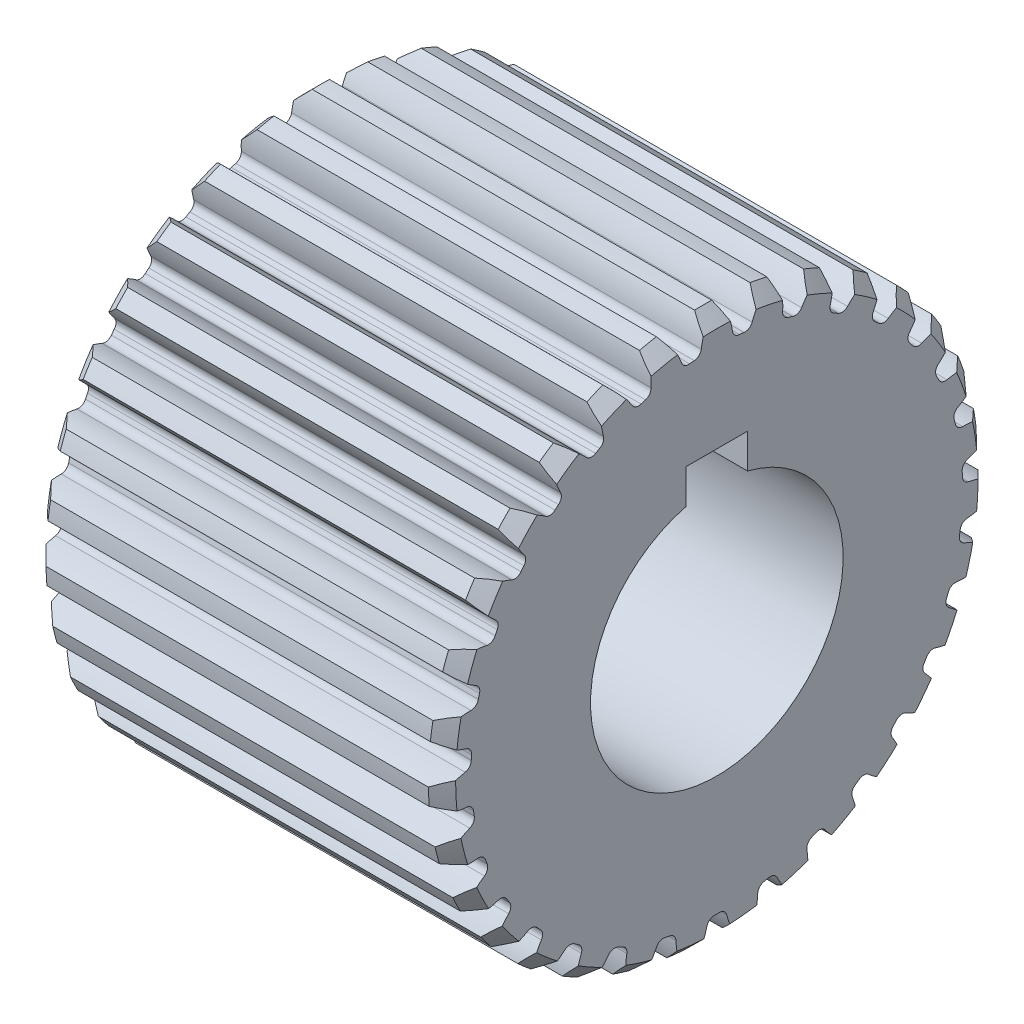
SolidWorks part; units mm, degrees
ref_plane "Front" through (0, 0, 0) normal (0, 0, 1) x (1, 0, 0)
ref_plane "Top" through (0, 0, 0) normal (0, 1, 0) x (1, 0, 0)
ref_plane "Right" through (0, 0, 0) normal (1, 0, 0) x (0, 0, -1)
sketch "Sketch1" plane through (0, 0, 0) normal (0, 0, 1) x (1, 0, 0)
  line L1 (31.1495, 18.25) -> (31.1495, 38.25)
  line L2 (31.1495, 38.25) -> (29.1495, 40.25)
  line L3 (29.1495, 40.25) -> (-26.8505, 40.25)
  line L4 (-26.8505, 40.25) -> (-28.8505, 38.25)
  line L5 (-28.8505, 38.25) -> (-28.8505, 18.25)
  line L6 (-28.8505, 18.25) -> (-28.8505, 0)
  line L7 (-28.8505, 0) -> (31.1495, 0)
  line L8 (31.1495, 0) -> (31.1495, 18.25)
  dimension "D2" = 40.25
  dimension "D3" = 60
  dimension "D4" = 56
  dimension "D5" = 2
  dimension "D6" = 2
  dimension "D7" = 2
revolve "Revolve1" add sketch "Sketch1" angle 360 about L7
sketch "Sketch2" plane through (0, 0, 0) normal (0, 0, 1) x (1, 0, 0)
  line L0 (0, 0) -> (44.1495, 0)
  line L1 (44.1495, 0) -> (44.1495, 19)
  line L2 (44.1495, 19) -> (-36.766, 19)
  line L3 (-36.766, 19) -> (-36.766, 0)
  line L4 (-36.766, 0) -> (0, 0)
  line L5 (0, 0) -> (0.5684, -0.1453)
  dimension "D1" = 19
revolve "Cut-Revolve1" cut sketch "Sketch2" angle 360 about L4
sketch "Sketch3" plane through (-28.8505, 0, 0) normal (-1, 0, 0) x (0, 0, 1)
  circle A0 centre (0, 0) radius 40.25 construction
  circle A1 centre (0, 0) radius 40.25
sketch "Sketch4" plane through (-28.8505, 0, 0) normal (-1, 0, 0) x (0, 0, 1)
  line L0 (0, 0) -> (0, 50.4222) construction
  circle A0 centre (0, 0) radius 40.25 construction
  arc A1 (1.2604, 40.2303) -> (-1.2604, 40.2303) centre (0, 0) ccw
  arc A2 (1.9993, 38.6984) -> (1.8415, 38.7062) centre (0, 0) ccw
  arc A3 (6.8637, 39.6605) -> (5.1716, 36.4916) centre (17.2742, 32.0653) ccw
  arc A4 (1.8415, 38.7062) -> (1.9993, 38.6984) centre (0, 0) cw
  arc A5 (9.3329, 39.153) -> (6.8637, 39.6605) centre (0, 0) ccw
  arc A6 (1.2604, 40.2303) -> (2.2799, 36.7857) centre (-10.4659, 34.8861) cw
  arc A7 (-1.2604, 40.2303) -> (-2.2799, 36.7857) centre (10.4659, 34.8861) ccw
  arc A8 (9.3329, 39.153) -> (9.6382, 35.5737) centre (-3.2291, 36.2788) cw
  arc A9 (3.9794, 35.7794) -> (5.1716, 36.4916) centre (4.1366, 36.8702) ccw
  arc A10 (10.453, 34.449) -> (9.6382, 35.5737) centre (10.7386, 35.5134) cw
  arc A11 (14.7068, 37.4669) -> (12.4115, 34.7036) centre (23.3753, 27.9316) ccw
  arc A12 (17.0233, 36.4729) -> (14.7068, 37.4669) centre (0, 0) ccw
  arc A13 (17.0233, 36.4729) -> (16.6018, 32.9054) centre (4.1398, 36.1862) cw
  arc A14 (11.1002, 34.2459) -> (12.4115, 34.7036) centre (11.4738, 35.2828) ccw
  arc A15 (17.1735, 31.6397) -> (16.6018, 32.9054) centre (17.6676, 32.6248) cw
  arc A16 (21.9478, 33.7395) -> (19.1432, 31.4948) centre (28.5194, 22.6544) ccw
  arc A17 (24.0167, 32.2995) -> (21.9478, 33.7395) centre (0, 0) ccw
  arc A18 (24.0167, 32.2995) -> (22.8858, 28.8899) centre (11.3393, 34.6121) cw
  arc A19 (17.7667, 31.3105) -> (19.1432, 31.4948) centre (18.3413, 32.2509) ccw
  arc A20 (23.191, 27.535) -> (22.8858, 28.8899) centre (23.8733, 28.4005) cw
  arc A21 (28.2903, 28.6308) -> (25.0912, 26.9966) centre (32.4959, 16.4498) ccw
  arc A22 (30.027, 26.8038) -> (28.2903, 28.6308) centre (0, 0) ccw
  arc A23 (30.027, 26.8038) -> (28.2328, 23.6916) centre (18.0746, 31.621) cw
  arc A24 (23.7057, 27.0931) -> (25.0912, 26.9966) centre (24.4579, 27.8986) ccw
  arc A25 (28.259, 22.3031) -> (28.2328, 23.6916) centre (29.1016, 23.0135) cw
  arc A26 (33.4745, 22.35) -> (30.012, 21.3932) centre (35.142, 9.5717) ccw
  arc A27 (34.8079, 20.2108) -> (33.4745, 22.35) centre (0, 0) ccw
  arc A28 (34.8079, 20.2108) -> (32.424, 17.5234) centre (24.0698, 27.3354) cw
  arc A29 (28.6743, 21.7666) -> (30.012, 21.3932) centre (29.5732, 22.4042) ccw
  arc A30 (32.1701, 16.158) -> (32.424, 17.5234) centre (33.1384, 16.6843) cw
  arc A31 (37.2883, 15.1541) -> (33.704, 14.9139) centre (36.3494, 2.3017) ccw
  arc A32 (38.1637, 12.7903) -> (37.2883, 15.1541) centre (0, 0) ccw
  arc A33 (38.1637, 12.7903) -> (35.2877, 10.6378) centre (29.0797, 21.9306) cw
  arc A34 (32.4689, 15.549) -> (33.704, 14.9139) centre (33.4778, 15.9925) ccw
  arc A35 (34.7642, 9.3515) -> (35.2877, 10.6378) centre (35.8186, 9.6721) cw
  arc A36 (39.5755, 7.3378) -> (36.0163, 7.824) centre (36.0687, -5.0625) ccw
  arc A37 (39.9572, 4.8461) -> (39.5755, 7.3378) centre (0, 0) ccw
  arc A38 (39.9572, 4.8461) -> (36.7067, 3.3167) centre (32.899, 15.628) cw
  arc A39 (34.9342, 8.6947) -> (36.0163, 7.824) centre (36.0118, 8.9261) ccw
  arc A40 (35.935, 2.1621) -> (36.7067, 3.3167) centre (37.0324, 2.2638) cw
  arc A41 (40.2425, -0.7789) -> (36.854, 0.4139) centre (34.3113, -12.2194) ccw
  arc A42 (40.1148, -3.2964) -> (40.2425, -0.7789) centre (0, 0) ccw
  arc A43 (40.1148, -3.2964) -> (36.623, -4.1402) centre (35.3715, 8.6855) cw
  arc A44 (35.9694, 1.4845) -> (36.854, 0.4139) centre (37.0714, 1.4943) ccw
  arc A45 (35.6346, -5.1159) -> (36.623, -4.1402) centre (36.73, -5.2371) cw
  arc A46 (39.2619, -8.8637) -> (36.1829, -7.0133) centre (31.1492, -18.8761) ccw
  arc A47 (38.6301, -11.3039) -> (39.2619, -8.8637) centre (0, 0) ccw
  arc A48 (38.6301, -11.3039) -> (35.0399, -11.4276) centre (36.3958, 1.3875) cw
  arc A49 (35.5319, -5.7864) -> (36.1829, -7.0133) centre (36.6134, -5.9987) ccw
  arc A50 (33.8754, -12.1844) -> (35.0399, -11.4276) centre (34.924, -12.5236) cw
  arc A51 (36.674, -16.5856) -> (34.0304, -14.1533) centre (26.7118, -24.76) ccw
  arc A52 (35.5639, -18.8487) -> (36.674, -16.5856) centre (0, 0) ccw
  arc A53 (35.5639, -18.8487) -> (32.0223, -18.2472) centre (35.9301, -5.9673) cw
  arc A54 (33.6398, -12.8205) -> (34.0304, -14.1533) centre (34.6563, -13.2462) ccw
  arc A55 (30.7293, -18.754) -> (32.0223, -18.2472) centre (31.6881, -19.2973) cw
  arc A56 (32.5846, -23.6285) -> (30.4848, -20.7138) centre (21.1809, -29.6302) ccw
  arc A57 (31.0416, -25.6219) -> (32.5846, -23.6285) centre (0, 0) ccw
  arc A58 (31.0416, -25.6219) -> (27.6937, -24.3197) centre (33.9934, -13.0778) cw
  arc A59 (30.3704, -19.3297) -> (30.4848, -20.7138) centre (31.2805, -19.9513) ccw
  arc A60 (26.3251, -24.5559) -> (27.6937, -24.3197) centre (27.1549, -25.2811) cw
  arc A61 (27.1612, -29.7041) -> (25.6911, -26.4264) centre (14.7828, -33.2874) ccw
  arc A62 (25.2486, -31.346) -> (27.1612, -29.7041) centre (0, 0) ccw
  arc A63 (25.2486, -31.346) -> (22.2313, -29.3965) centre (30.665, -19.6529) cw
  arc A64 (25.8577, -25.0476) -> (25.6911, -26.4264) centre (26.624, -25.8396) ccw
  arc A65 (20.8431, -29.3524) -> (22.2313, -29.3965) centre (21.51, -30.2298) cw
  arc A66 (20.6258, -34.5635) -> (19.8456, -31.057) centre (7.7795, -35.5817) ccw
  arc A67 (18.4218, -35.7869) -> (20.6258, -34.5635) centre (0, 0) ccw
  arc A68 (18.4218, -35.7869) -> (15.8587, -33.2699) centre (26.0812, -25.4235) cw
  arc A69 (20.2863, -29.7399) -> (19.8456, -31.057) centre (20.8776, -30.67) ccw
  arc A70 (14.5079, -32.9472) -> (15.8587, -33.2699) centre (14.9845, -33.941) cw
  arc A71 (13.246, -38.008) -> (13.1877, -34.4162) centre (0.4577, -36.4193) ccw
  arc A72 (10.8409, -38.7626) -> (13.246, -38.008) centre (0, 0) ccw
  arc A73 (10.8409, -38.7626) -> (8.8369, -35.7812) centre (20.4296, -30.1531) cw
  arc A74 (13.8845, -33.2148) -> (13.1877, -34.4162) centre (14.2764, -34.2448) ccw
  arc A75 (7.5787, -35.1932) -> (8.8369, -35.7812) centre (7.8455, -36.2625) cw
  arc A76 (5.3239, -39.8963) -> (5.9898, -36.3663) centre (-6.8828, -35.766) ccw
  arc A77 (2.8161, -40.1514) -> (5.3239, -39.8963) centre (0, 0) ccw
  arc A78 (2.8161, -40.1514) -> (1.4533, -36.8276) centre (13.9416, -33.6483) cw
  arc A79 (6.9142, -35.3298) -> (5.9898, -36.3663) centre (7.0907, -36.4176) ccw
  arc A80 (0.3392, -35.9984) -> (1.4533, -36.8276) centre (0.3853, -37.0995) cw
  arc A81 (-2.8161, -40.1514) -> (-1.4533, -36.8276) centre (-13.9416, -33.6483) ccw
  arc A82 (-5.3239, -39.8963) -> (-2.8161, -40.1514) centre (0, 0) ccw
  arc A83 (-5.3239, -39.8963) -> (-5.9898, -36.3663) centre (6.8828, -35.766) cw
  arc A84 (-0.3392, -35.9984) -> (-1.4533, -36.8276) centre (-0.3853, -37.0995) ccw
  arc A85 (-6.9142, -35.3298) -> (-5.9898, -36.3663) centre (-7.0907, -36.4176) cw
  arc A86 (-10.8409, -38.7626) -> (-8.8369, -35.7812) centre (-20.4296, -30.1531) ccw
  arc A87 (-13.246, -38.008) -> (-10.8409, -38.7626) centre (0, 0) ccw
  arc A88 (-13.246, -38.008) -> (-13.1877, -34.4162) centre (-0.4577, -36.4193) cw
  arc A89 (-7.5787, -35.1932) -> (-8.8369, -35.7812) centre (-7.8455, -36.2625) ccw
  arc A90 (-13.8845, -33.2148) -> (-13.1877, -34.4162) centre (-14.2764, -34.2448) cw
  arc A91 (-18.4218, -35.7869) -> (-15.8587, -33.2699) centre (-26.0812, -25.4235) ccw
  arc A92 (-20.6258, -34.5635) -> (-18.4218, -35.7869) centre (0, 0) ccw
  arc A93 (-20.6258, -34.5635) -> (-19.8456, -31.057) centre (-7.7795, -35.5817) cw
  arc A94 (-14.5079, -32.9472) -> (-15.8587, -33.2699) centre (-14.9845, -33.941) ccw
  arc A95 (-20.2863, -29.7399) -> (-19.8456, -31.057) centre (-20.8776, -30.67) cw
  arc A96 (-25.2486, -31.346) -> (-22.2313, -29.3965) centre (-30.665, -19.6529) ccw
  arc A97 (-27.1612, -29.7041) -> (-25.2486, -31.346) centre (0, 0) ccw
  arc A98 (-27.1612, -29.7041) -> (-25.6911, -26.4264) centre (-14.7828, -33.2874) cw
  arc A99 (-20.8431, -29.3524) -> (-22.2313, -29.3965) centre (-21.51, -30.2298) ccw
  arc A100 (-25.8577, -25.0476) -> (-25.6911, -26.4264) centre (-26.624, -25.8396) cw
  arc A101 (-31.0416, -25.6219) -> (-27.6937, -24.3197) centre (-33.9934, -13.0778) ccw
  arc A102 (-32.5846, -23.6285) -> (-31.0416, -25.6219) centre (0, 0) ccw
  arc A103 (-32.5846, -23.6285) -> (-30.4848, -20.7138) centre (-21.1809, -29.6302) cw
  arc A104 (-26.3251, -24.5559) -> (-27.6937, -24.3197) centre (-27.1549, -25.2811) ccw
  arc A105 (-30.3704, -19.3297) -> (-30.4848, -20.7138) centre (-31.2805, -19.9513) cw
  arc A106 (-35.5639, -18.8487) -> (-32.0223, -18.2472) centre (-35.9301, -5.9673) ccw
  arc A107 (-36.674, -16.5856) -> (-35.5639, -18.8487) centre (0, 0) ccw
  arc A108 (-36.674, -16.5856) -> (-34.0304, -14.1533) centre (-26.7118, -24.76) cw
  arc A109 (-30.7293, -18.754) -> (-32.0223, -18.2472) centre (-31.6881, -19.2973) ccw
  arc A110 (-33.6398, -12.8205) -> (-34.0304, -14.1533) centre (-34.6563, -13.2462) cw
  arc A111 (-38.6301, -11.3039) -> (-35.0399, -11.4276) centre (-36.3958, 1.3875) ccw
  arc A112 (-39.2619, -8.8637) -> (-38.6301, -11.3039) centre (0, 0) ccw
  arc A113 (-39.2619, -8.8637) -> (-36.1829, -7.0133) centre (-31.1492, -18.8761) cw
  arc A114 (-33.8754, -12.1844) -> (-35.0399, -11.4276) centre (-34.924, -12.5236) ccw
  arc A115 (-35.5319, -5.7864) -> (-36.1829, -7.0133) centre (-36.6134, -5.9987) cw
  arc A116 (-40.1148, -3.2964) -> (-36.623, -4.1402) centre (-35.3715, 8.6855) ccw
  arc A117 (-40.2425, -0.7789) -> (-40.1148, -3.2964) centre (0, 0) ccw
  arc A118 (-40.2425, -0.7789) -> (-36.854, 0.4139) centre (-34.3113, -12.2194) cw
  arc A119 (-35.6346, -5.1159) -> (-36.623, -4.1402) centre (-36.73, -5.2371) ccw
  arc A120 (-35.9694, 1.4845) -> (-36.854, 0.4139) centre (-37.0714, 1.4943) cw
  arc A121 (-39.9572, 4.8461) -> (-36.7067, 3.3167) centre (-32.899, 15.628) ccw
  arc A122 (-39.5755, 7.3378) -> (-39.9572, 4.8461) centre (0, 0) ccw
  arc A123 (-39.5755, 7.3378) -> (-36.0163, 7.824) centre (-36.0687, -5.0625) cw
  arc A124 (-35.935, 2.1621) -> (-36.7067, 3.3167) centre (-37.0324, 2.2638) ccw
  arc A125 (-34.9342, 8.6947) -> (-36.0163, 7.824) centre (-36.0118, 8.9261) cw
  arc A126 (-38.1637, 12.7903) -> (-35.2877, 10.6378) centre (-29.0797, 21.9306) ccw
  arc A127 (-37.2883, 15.1541) -> (-38.1637, 12.7903) centre (0, 0) ccw
  arc A128 (-37.2883, 15.1541) -> (-33.704, 14.9139) centre (-36.3494, 2.3017) cw
  arc A129 (-34.7642, 9.3515) -> (-35.2877, 10.6378) centre (-35.8186, 9.6721) ccw
  arc A130 (-32.4689, 15.549) -> (-33.704, 14.9139) centre (-33.4778, 15.9925) cw
  arc A131 (-34.8079, 20.2108) -> (-32.424, 17.5234) centre (-24.0698, 27.3354) ccw
  arc A132 (-33.4745, 22.35) -> (-34.8079, 20.2108) centre (0, 0) ccw
  arc A133 (-33.4745, 22.35) -> (-30.012, 21.3932) centre (-35.142, 9.5717) cw
  arc A134 (-32.1701, 16.158) -> (-32.424, 17.5234) centre (-33.1384, 16.6843) ccw
  arc A135 (-28.6743, 21.7666) -> (-30.012, 21.3932) centre (-29.5732, 22.4042) cw
  arc A136 (-30.027, 26.8038) -> (-28.2328, 23.6916) centre (-18.0746, 31.621) ccw
  arc A137 (-28.2903, 28.6308) -> (-30.027, 26.8038) centre (0, 0) ccw
  arc A138 (-28.2903, 28.6308) -> (-25.0912, 26.9966) centre (-32.4959, 16.4498) cw
  arc A139 (-28.259, 22.3031) -> (-28.2328, 23.6916) centre (-29.1016, 23.0135) ccw
  arc A140 (-23.7057, 27.0931) -> (-25.0912, 26.9966) centre (-24.4579, 27.8986) cw
  arc A141 (-24.0167, 32.2995) -> (-22.8858, 28.8899) centre (-11.3393, 34.6121) ccw
  arc A142 (-21.9478, 33.7395) -> (-24.0167, 32.2995) centre (0, 0) ccw
  arc A143 (-21.9478, 33.7395) -> (-19.1432, 31.4948) centre (-28.5194, 22.6544) cw
  arc A144 (-23.191, 27.535) -> (-22.8858, 28.8899) centre (-23.8733, 28.4005) ccw
  arc A145 (-17.7667, 31.3105) -> (-19.1432, 31.4948) centre (-18.3413, 32.2509) cw
  arc A146 (-17.0233, 36.4729) -> (-16.6018, 32.9054) centre (-4.1398, 36.1862) ccw
  arc A147 (-14.7068, 37.4669) -> (-17.0233, 36.4729) centre (0, 0) ccw
  arc A148 (-14.7068, 37.4669) -> (-12.4115, 34.7036) centre (-23.3753, 27.9316) cw
  arc A149 (-17.1735, 31.6397) -> (-16.6018, 32.9054) centre (-17.6676, 32.6248) ccw
  arc A150 (-11.1002, 34.2459) -> (-12.4115, 34.7036) centre (-11.4738, 35.2828) cw
  arc A151 (-9.3329, 39.153) -> (-9.6382, 35.5737) centre (3.2291, 36.2788) ccw
  arc A152 (-6.8637, 39.6605) -> (-9.3329, 39.153) centre (0, 0) ccw
  arc A153 (-6.8637, 39.6605) -> (-5.1716, 36.4916) centre (-17.2742, 32.0653) cw
  arc A154 (-10.453, 34.449) -> (-9.6382, 35.5737) centre (-10.7386, 35.5134) ccw
  arc A155 (-3.9794, 35.7794) -> (-5.1716, 36.4916) centre (-4.1366, 36.8702) cw
  arc A156 (-3.3044, 35.848) -> (-3.9794, 35.7794) centre (0, 0) ccw
  arc A157 (3.9794, 35.7794) -> (3.3044, 35.848) centre (0, 0) ccw
  arc A158 (11.1002, 34.2459) -> (10.453, 34.449) centre (0, 0) ccw
  arc A159 (17.7667, 31.3105) -> (17.1735, 31.6397) centre (0, 0) ccw
  arc A160 (23.7057, 27.0931) -> (23.191, 27.535) centre (0, 0) ccw
  arc A161 (28.6743, 21.7666) -> (28.259, 22.3031) centre (0, 0) ccw
  arc A162 (32.4689, 15.549) -> (32.1701, 16.158) centre (0, 0) ccw
  arc A163 (34.9342, 8.6947) -> (34.7642, 9.3515) centre (0, 0) ccw
  arc A164 (35.9694, 1.4845) -> (35.935, 2.1621) centre (0, 0) ccw
  arc A165 (35.5319, -5.7864) -> (35.6346, -5.1159) centre (0, 0) ccw
  arc A166 (33.6398, -12.8205) -> (33.8754, -12.1844) centre (0, 0) ccw
  arc A167 (30.3704, -19.3297) -> (30.7293, -18.754) centre (0, 0) ccw
  arc A168 (25.8577, -25.0476) -> (26.3251, -24.5559) centre (0, 0) ccw
  arc A169 (20.2863, -29.7399) -> (20.8431, -29.3524) centre (0, 0) ccw
  arc A170 (13.8845, -33.2148) -> (14.5079, -32.9472) centre (0, 0) ccw
  arc A171 (6.9142, -35.3298) -> (7.5787, -35.1932) centre (0, 0) ccw
  arc A172 (-0.3392, -35.9984) -> (0.3392, -35.9984) centre (0, 0) ccw
  arc A173 (-7.5787, -35.1932) -> (-6.9142, -35.3298) centre (0, 0) ccw
  arc A174 (-14.5079, -32.9472) -> (-13.8845, -33.2148) centre (0, 0) ccw
  arc A175 (-20.8431, -29.3524) -> (-20.2863, -29.7399) centre (0, 0) ccw
  arc A176 (-26.3251, -24.5559) -> (-25.8577, -25.0476) centre (0, 0) ccw
  arc A177 (-30.7293, -18.754) -> (-30.3704, -19.3297) centre (0, 0) ccw
  arc A178 (-33.8754, -12.1844) -> (-33.6398, -12.8205) centre (0, 0) ccw
  arc A179 (-35.6346, -5.1159) -> (-35.5319, -5.7864) centre (0, 0) ccw
  arc A180 (-35.935, 2.1621) -> (-35.9694, 1.4845) centre (0, 0) ccw
  arc A181 (-34.7642, 9.3515) -> (-34.9342, 8.6947) centre (0, 0) ccw
  arc A182 (-32.1701, 16.158) -> (-32.4689, 15.549) centre (0, 0) ccw
  arc A183 (-28.259, 22.3031) -> (-28.6743, 21.7666) centre (0, 0) ccw
  arc A184 (-23.191, 27.535) -> (-23.7057, 27.0931) centre (0, 0) ccw
  arc A185 (-10.453, 34.449) -> (-11.1002, 34.2459) centre (0, 0) ccw
  arc A186 (-17.1735, 31.6397) -> (-17.7667, 31.3105) centre (0, 0) ccw
  arc A191 (-3.3044, 35.848) -> (-2.2799, 36.7857) centre (-3.37, 36.9482) ccw
  arc A192 (3.3044, 35.848) -> (2.2799, 36.7857) centre (3.37, 36.9482) cw
  point P314 (0, 0)
  point P318 (0, 0)
  dimension "D1" = 77.5
  dimension "D2" = 72
  dimension "D8" = 1.1021
extrude "Cut-Extrude6" cut sketch "Sketch4" against normal up to next (60 mm away) flip side to cut
sketch "Sketch5" plane through (-28.8505, 0, 0) normal (-1, 0, 0) x (0, 0, 1)
  line L1 (-4.5, 0) -> (4.5, 0)
  line L2 (-4.5, 0) -> (-4.5, 23)
  line L3 (-4.5, 23) -> (4.5, 23)
  line L4 (4.5, 0) -> (4.5, 23)
  circle A0 centre (0, 0) radius 19 construction
  circle A1 centre (0, 0) radius 19
  dimension "D1" = 23
  dimension "D2" = 9
  dimension "D3" = 4.5
extrude "Cut-Extrude7" cut sketch "Sketch5" against normal up to next contours L4 L3 L2 L1
sketch "Sketch7" plane through (-28.8505, 0, 0) normal (-1, 0, 0) x (0, 0, 1)
  line L0 (4.5, 18.4594) -> (4.5, 17.9444)
  line L1 (-4.5, 18.4594) -> (-4.5, 17.9444)
  arc A0 (-4.5, 17.9444) -> (4.5, 17.9444) centre (0, 0) ccw
  arc A1 (-4.5, 18.4594) -> (4.5, 18.4594) centre (0, 0) ccw
  dimension "D1" = 37
extrude "Boss-Extrude1" add sketch "Sketch7" against normal up to surface (60 mm away)
scale "Scale 1" bodies to scale 107 scale about centroid uniform scaling yes scale factor 1.875
